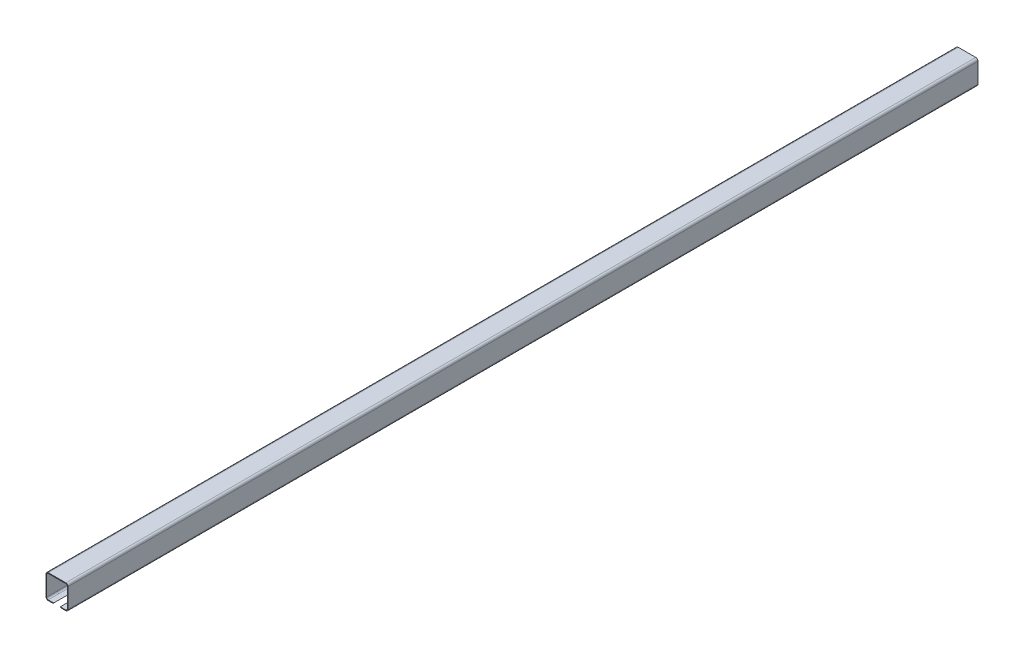
SolidWorks part; units mm, degrees
ref_plane "Front Plane" through (0, 0, 0) normal (0, 0, 1) x (1, 0, 0)
ref_plane "Top Plane" through (0, 0, 0) normal (0, 1, 0) x (1, 0, 0)
ref_plane "Right Plane" through (0, 0, 0) normal (1, 0, 0) x (0, 0, -1)
other "Configuration Table"
sketch "Sketch1" plane through (0, 0, 0) normal (0, 0, 1) x (1, 0, 0)
  line L0 (0, 55) -> (0, -114.6613) construction
  line L1 (-40, 55) -> (0, 55)
  line L2 (-50, 45) -> (-50, -45)
  line L3 (-40, -55) -> (-18, -55)
  line L4 (50, 45) -> (50, -45)
  line L5 (-50, 55) -> (50, -55) construction
  line L6 (-50, -55) -> (50, 55) construction
  line L9 (18, -55) -> (40, -55)
  line L11 (0, 55) -> (40, 55)
  line L14 (15, -52) -> (40, -52)
  line L15 (47, 45) -> (47, -45)
  line L16 (0, 52) -> (40, 52)
  line L19 (-40, 52) -> (0, 52)
  line L20 (-47, 45) -> (-47, -45)
  line L21 (-40, -52) -> (-15, -52)
  line L25 (2, 85.672) -> (2, 52) construction
  line L26 (-2, 85.672) -> (-2, 52) construction
  line L27 (-5, 83.72) -> (-5, 55) construction
  line L28 (5, 83.72) -> (5, 55) construction
  line L29 (5, 55) -> (40, 55) construction
  line L30 (2, 52) -> (40, 52) construction
  line L31 (-40, 52) -> (-2, 52) construction
  line L32 (-40, 55) -> (-5, 55) construction
  line L33 (18, -92.3951) -> (18, -55) construction
  line L34 (15, -92.3951) -> (15, -52) construction
  line L35 (-18, -92.3951) -> (-18, -55) construction
  line L36 (-15, -92.3951) -> (-15, -52) construction
  line L37 (-15, -52) -> (-18, -55)
  line L38 (15, -52) -> (18, -55)
  arc A2 (-50, -45) -> (-40, -55) centre (-40, -45) ccw
  arc A4 (40, -55) -> (50, -45) centre (40, -45) ccw
  arc A5 (40, 55) -> (50, 45) centre (40, 45) cw
  arc A6 (-40, 55) -> (-50, 45) centre (-40, 45) ccw
  arc A8 (40, -52) -> (47, -45) centre (40, -45) ccw
  arc A9 (40, 52) -> (47, 45) centre (40, 45) cw
  arc A11 (-40, 52) -> (-47, 45) centre (-40, 45) ccw
  arc A12 (-47, -45) -> (-40, -52) centre (-40, -45) ccw
  arc A14 (2, 85.672) -> (-2, 85.672) centre (0, 92.3802) ccw construction
  arc A15 (5, 83.72) -> (-5, 83.72) centre (0, 92.3802) ccw construction
  arc A16 (29.5037, -90.0943) -> (18, -92.3951) centre (23.9819, -92.3951) cw construction
  arc A17 (32.2729, -88.9405) -> (15, -92.3951) centre (23.9819, -92.3951) cw construction
  arc A18 (-29.5037, -90.0943) -> (-18, -92.3951) centre (-23.9819, -92.3951) ccw construction
  arc A19 (-32.2729, -88.9405) -> (-15, -92.3951) centre (-23.9819, -92.3951) ccw construction
  point P0 (0, 0)
  dimension "D6" = 10
  dimension "D1" = 100
  dimension "D2" = 110
extrude "Boss-Extrude1" add sketch "Sketch1" along normal blind 4135
